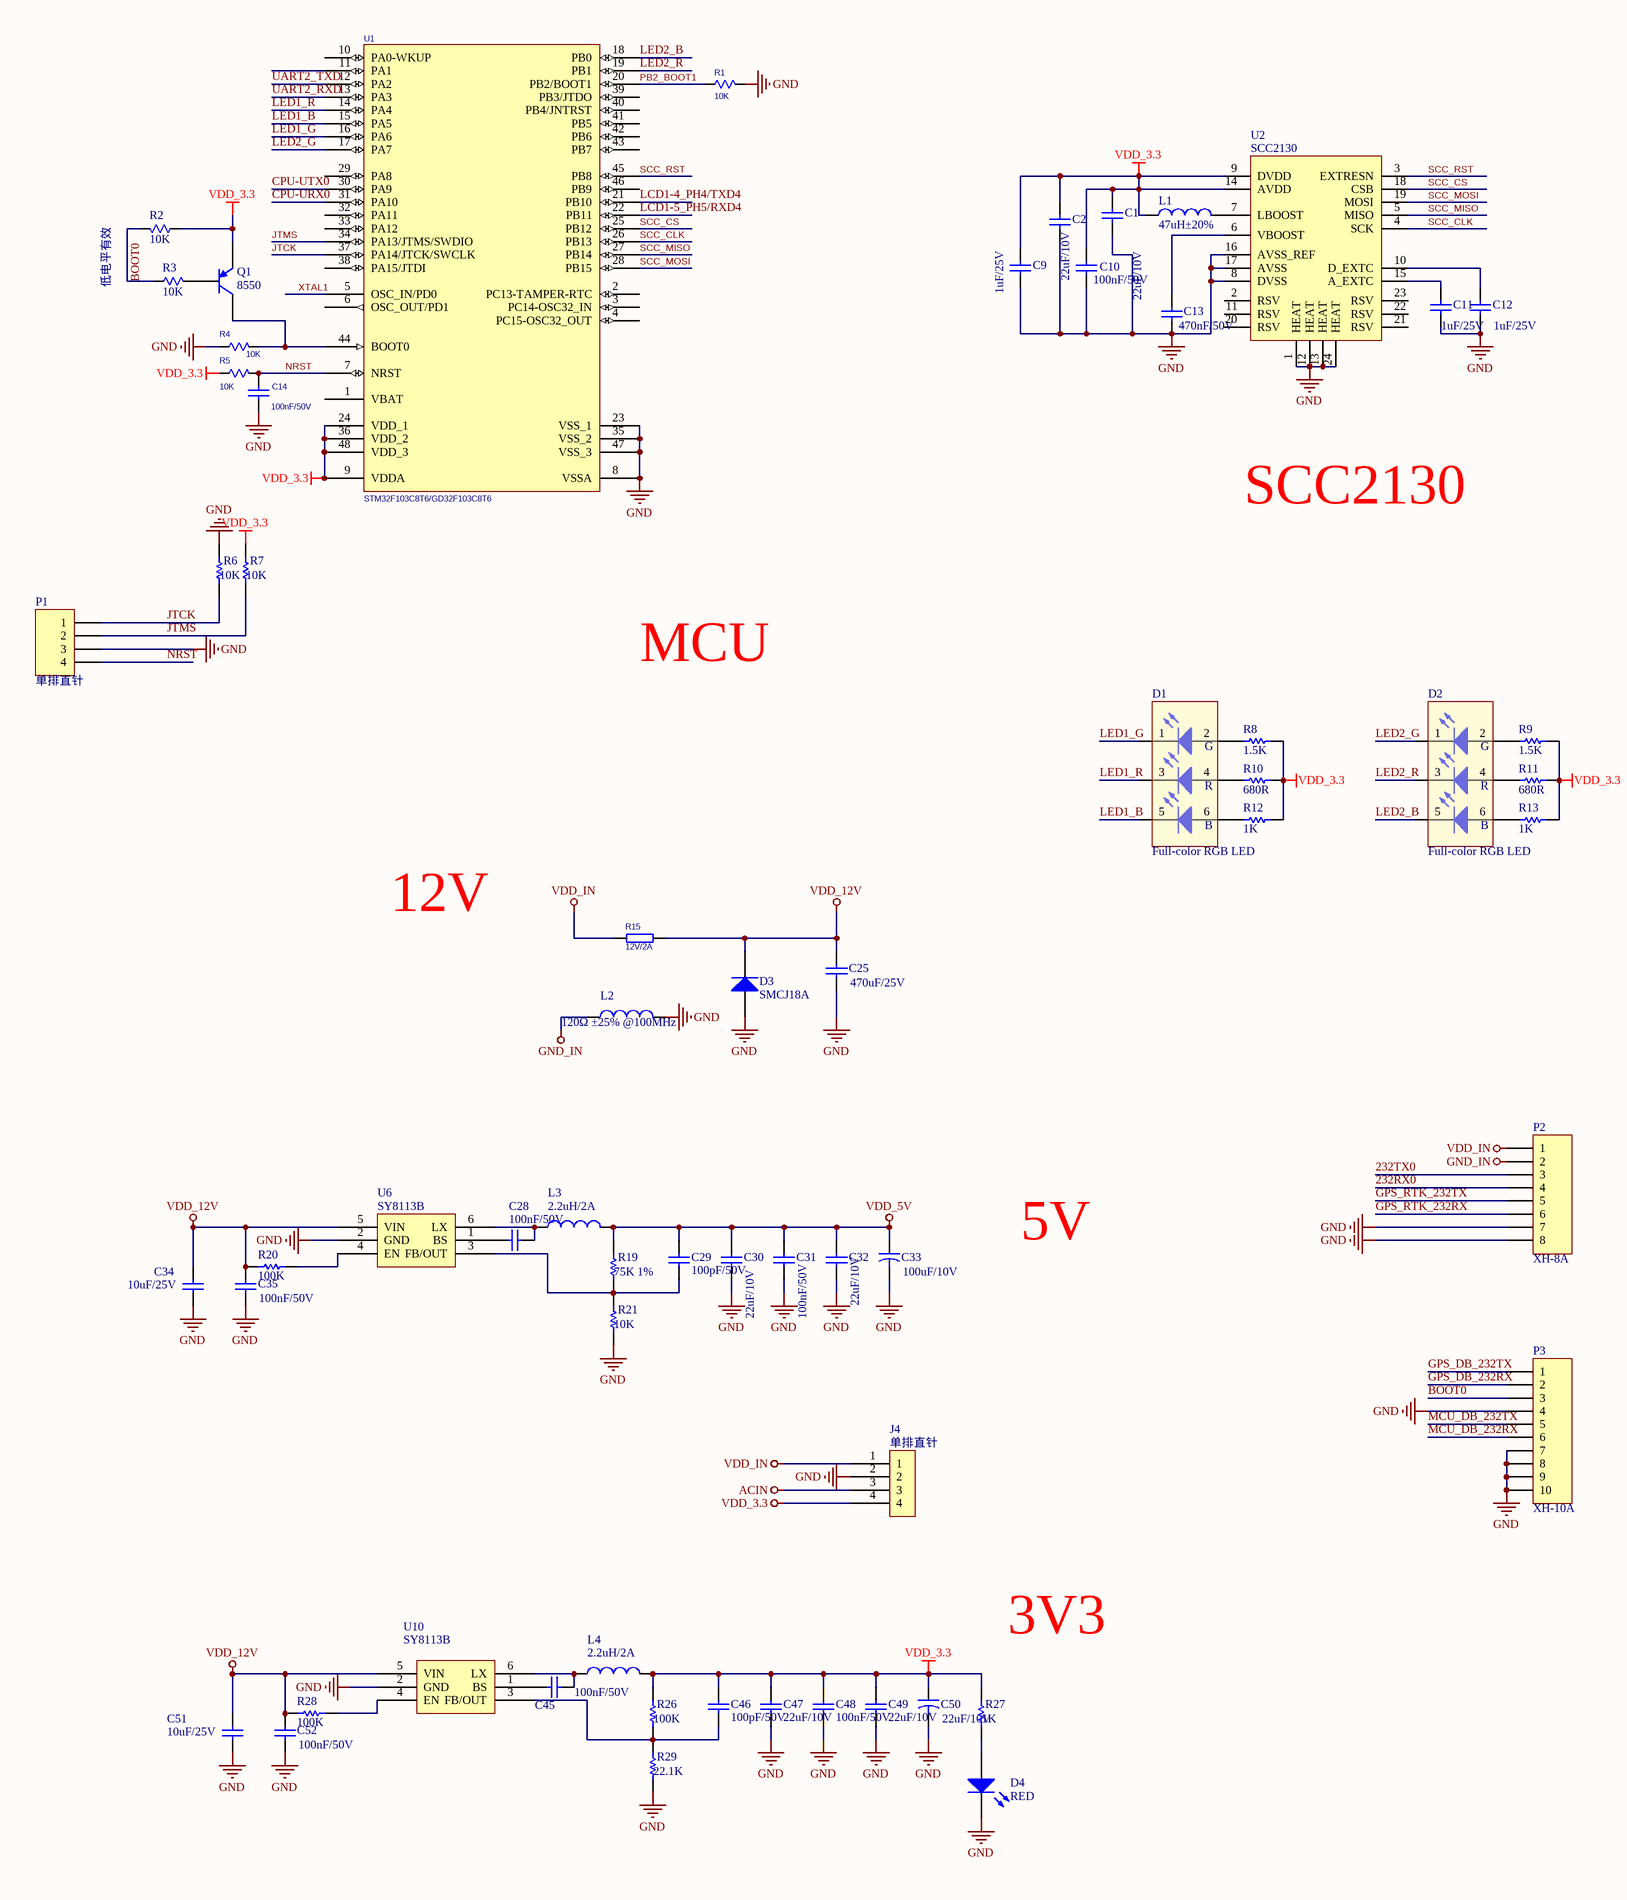
[diagram p0: MISC84436-2.SchDoc, left]
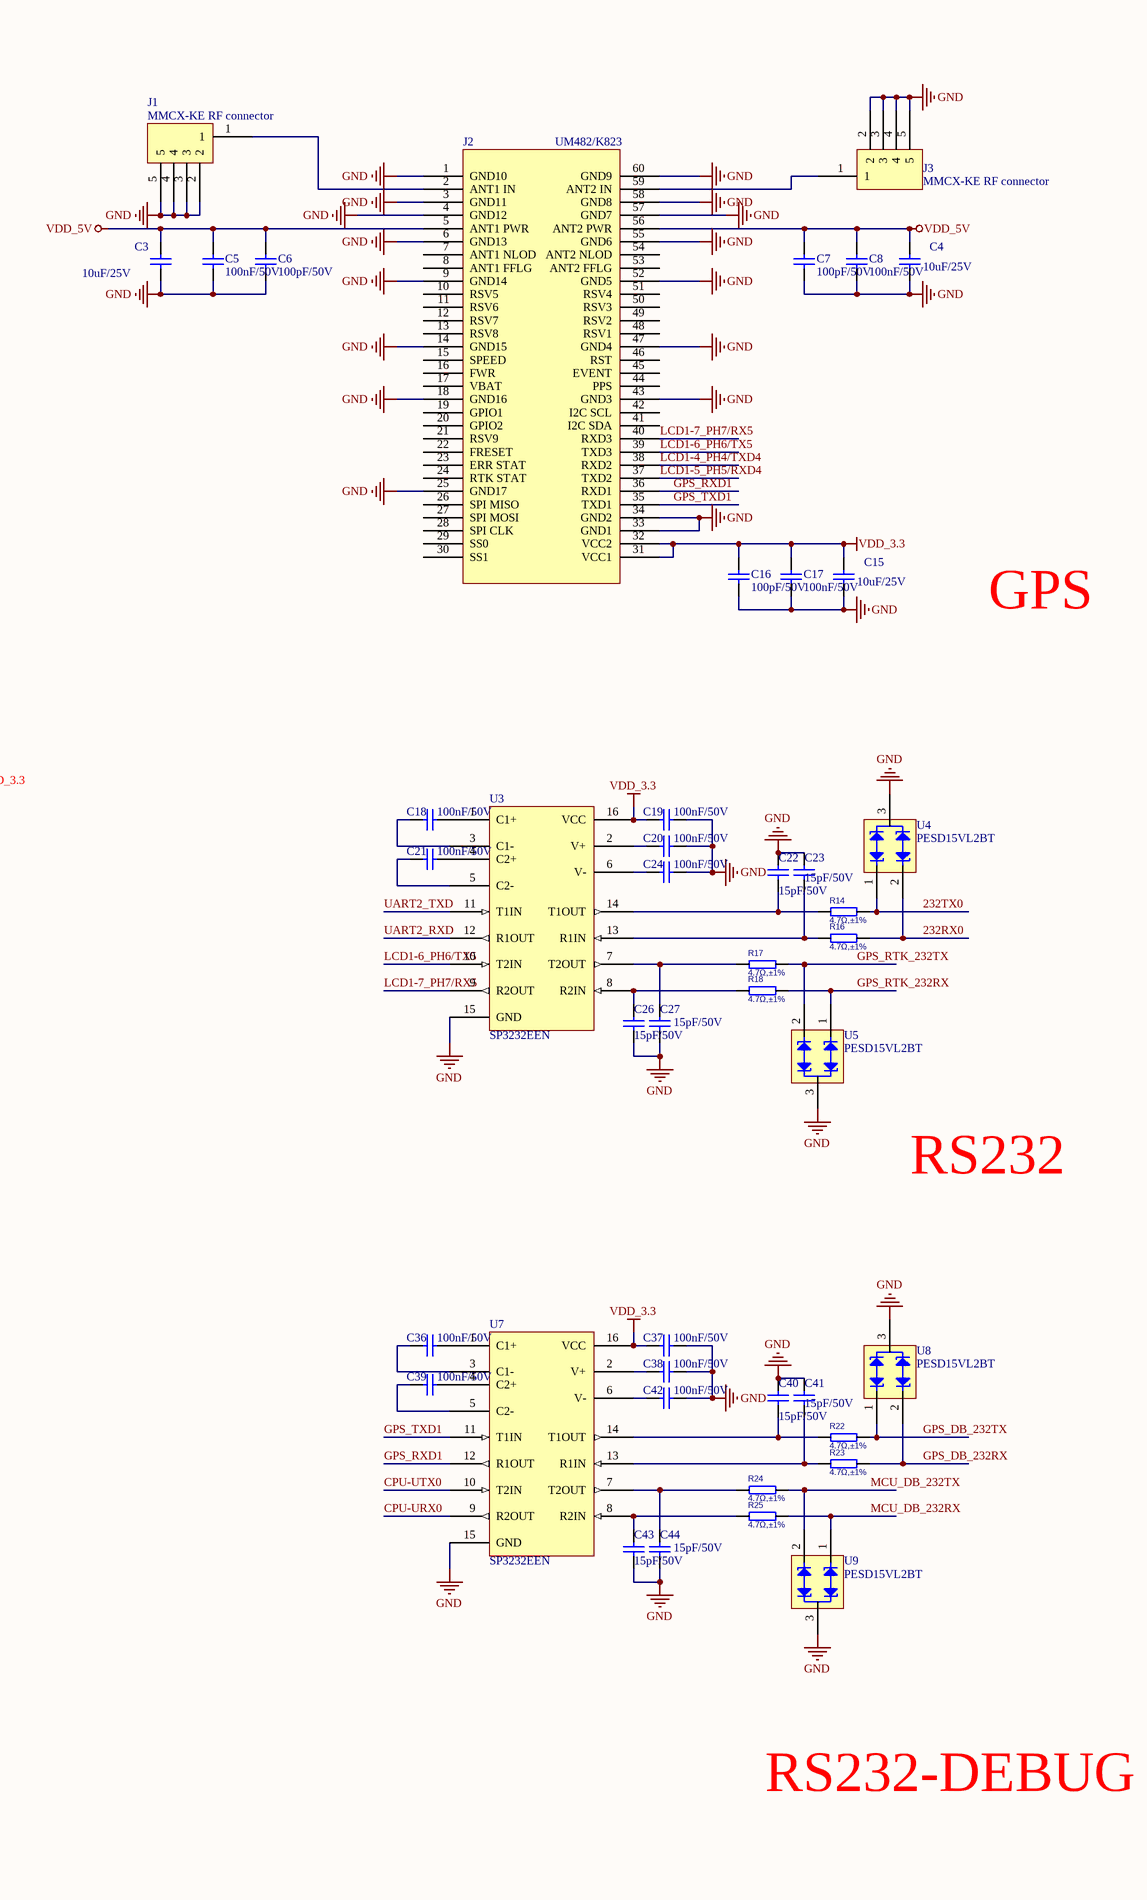
[diagram p1: MISC84436-2.SchDoc, right]
# Altium project MISC84436-3.PrjPcb
1 sheet, 107 parts. Net scope: global (net labels, ports and power ports of the same name join across sheets).
Board file: MISC84436.PcbDoc

## Sheet MISC84436-2.SchDoc
size A2

### Parts
C1  22uF/10V  [C0805]
C2  22uF/10V  [C0805]
C3  10uF/25V  [C0805]
C4  10uF/25V  [C0805]
C5  100nF/50V  [0603]
C6  100pF/50V  [0603]
C7  100pF/50V  [0603]
C8  100nF/50V  [0603]
C9  1uF/25V  [0603]
C10  100nF/50V  [0603]
C11  1uF/25V  [0603]
C12  1uF/25V  [0603]
C13  470nF/50V  [0603]
C14  100nF/50V  [0603]
C15  10uF/25V  [C0805]
C16  100pF/50V  [0603]
C17  100nF/50V  [0603]
C18  100nF/50V  [0603]
C19  100nF/50V  [0603]
C20  100nF/50V  [0603]
C21  100nF/50V  [0603]
C22  15pF/50V  [0603]
C23  15pF/50V  [0603]
C24  100nF/50V  [0603]
C25  470uF/25V  [CAP-TH_BD8.0-P3.50-D1.0-FD]
C26  15pF/50V  [0603]
C27  15pF/50V  [0603]
C28  100nF/50V  [0603]
C29  100pF/50V  [0603]
C30  22uF/10V  [C0805]
C31  100nF/50V  [0603]
C32  22uF/10V  [C0805]
C33  100uF/10V  [CAP-TH_BD5.0-P2.00-D0.8-FD]
C34  10uF/25V  [C0805]
C35  100nF/50V  [0603]
C36  100nF/50V  [0603]
C37  100nF/50V  [0603]
C38  100nF/50V  [0603]
C39  100nF/50V  [0603]
C40  15pF/50V  [0603]
C41  15pF/50V  [0603]
C42  100nF/50V  [0603]
C43  15pF/50V  [0603]
C44  15pF/50V  [0603]
C45  100nF/50V  [0603]
C46  100pF/50V  [0603]
C47  22uF/10V  [C0805]
C48  100nF/50V  [0603]
C49  22uF/10V  [C0805]
C50  22uF/10V  [C0805]
C51  10uF/25V  [C0805]
C52  100nF/50V  [0603]
D1  Full-color RGB LED  [RGB]
D2  Full-color RGB LED  [RGB]
D3  SMCJ18A  [SMC_L6.9-W5.9-LS7.9-RD]
D4  RED  [LED_0805]
J1  MMCX-KE RF connector  [MMCX-TH_ZC11.801KK]
J2  UM482/K823  [UM482/K823]
J3  MMCX-KE RF connector  [MMCX-TH_ZC11.801KK]
J4  单排直针  [HDR1X4]
L1  47uH±20%  [1210]
L2  120Ω ±25% @100MHz  [0603]
L3  2.2uH/2A  [IND-SMD_L4.0-W4.0]
L4  2.2uH/2A  [IND-SMD_L4.0-W4.0]
P1  单排直针  [HDR1X4]
P2  XH-8A  [CONN-TH_XH-8A]
P3  XH-10A  [CONN-TH_10P-P2.50_XH-10A]
Q1  8550  [SOT-23-SS8550]
R1  10K  [0603]
R2  10K  [0603]
R3  10K  [0603]
R4  10K  [0603]
R5  10K  [0603]
R6  10K  [0603]
R7  10K  [0603]
R8  1.5K  [0603]
R9  1.5K  [0603]
R10  680R  [0603]
R11  680R  [0603]
R12  1K  [0603]
R13  1K  [0603]
R14  4.7Ω,±1%  [0603]
R15  12V/2A  [1210]
R16  4.7Ω,±1%  [0603]
R17  4.7Ω,±1%  [0603]
R18  4.7Ω,±1%  [0603]
R19  75K 1%  [0603]
R20  100K  [0603]
R21  10K  [0603]
R22  4.7Ω,±1%  [0603]
R23  4.7Ω,±1%  [0603]
R24  4.7Ω,±1%  [0603]
R25  4.7Ω,±1%  [0603]
R26  100K  [0603]
R27  1K  [0603]
R28  100K  [0603]
R29  22.1K  [0603]
U1  STM32F103C8T6/GD32F103C8T6  [LQFP-48_L7.0-W7.0-P0.50-LS9.0-BL]
U2  SCC2130  [SCC2130D]
U3  SP3232EEN  [SOP16-6.6]
U4  PESD15VL2BT  [SOT-23]
U5  PESD15VL2BT  [SOT-23]
U6  SY8113B  [TSOT-23-6_L2.9-W1.6-P0.95-LS2.8-BR]
U7  SP3232EEN  [SOP16-6.6]
U8  PESD15VL2BT  [SOT-23]
U9  PESD15VL2BT  [SOT-23]
U10  SY8113B  [TSOT-23-6_L2.9-W1.6-P0.95-LS2.8-BR]

### Nets
ACIN: J4.3
GND: C1.2 C2.2 C3.1 C4.1 C5.2 C6.2 C7.1 C8.1 C9.2 C10.2 C11.2 C12.2 C13.2 C14.1 C15.1 C16.1 C17.1 C19.2 C20.2 C22.1 C23.1 C24.2 C25.2 C26.2 C27.2 C30.2 C31.2 C32.2 C33.2 C34.1 C35.1 C37.2 C38.2 C40.1 C41.1 C42.2 C43.2 C44.2 C47.2 C48.2 C49.2 C50.2 C51.1 C52.1 D3.1(A) D4.2(K) J1.2 J1.3 J1.4 J1.5 J2.1(GND10) J2.3(GND11) J2.4(GND12) J2.6(GND13) J2.9(GND14) J2.14(GND15) J2.18(GND16) J2.25(GND17) J2.33(GND1) J2.34(GND2) J2.43(GND3) J2.47(GND4) J2.52(GND5) J2.55(GND6) J2.57(GND7) J2.58(GND8) J2.60(GND9) J3.2 J3.3 J3.4 J3.5 J4.2 L2.2 P1.3 P2.7 P2.8 P3.4 P3.7 P3.8 P3.9 P3.10 R1.1 R4.1 R6.2 R21.1 R29.1 U1.8(VSSA) U1.23(VSS_1) U1.35(VSS_2) U1.47(VSS_3) U2.1(HEAT) U2.8(DVSS) U2.12(HEAT) U2.13(HEAT) U2.16(AVSS_REF) U2.17(AVSS) U2.24(HEAT) U3.15(GND) U4.3 U5.3 U6.2(GND) U7.15(GND) U8.3 U9.3 U10.2(GND)
GND_IN: L2.1 P2.2
VDD_3.3: C1.1 C2.1 C9.1 C10.1 C15.2 C16.2 C17.2 C19.1 C37.1 C46.1 C47.1 C48.1 C49.1 C50.1 J2.31(VCC1) J2.32(VCC2) J4.4 L1.1 L4.2 Q1.2(E) R2.2 R5.2 R7.2 R8.1 R9.1 R10.1 R11.1 R12.1 R13.1 R26.2 R27.2 U1.9(VDDA) U1.24(VDD_1) U1.36(VDD_2) U1.48(VDD_3) U2.9(DVDD) U2.14(AVDD) U3.16(VCC) U7.16(VCC)
VDD_5V: C3.2 C4.2 C5.1 C6.1 C7.2 C8.2 C29.1 C30.1 C31.1 C32.1 C33.1 J2.5(ANT1_PWR) J2.56(ANT2_PWR) L3.2 R19.2
VDD_12V: C25.1 C34.2 C35.2 C51.2 C52.2 D3.2(K) R15.1 R20.2 R28.2 U6.5(VIN) U10.5(VIN)
VDD_IN: J4.1 P2.1 R15.2
232RX0: P2.4 R16.1 U4.2
232TX0: P2.3 R14.1 U4.1
BOOT0: P3.3 R2.1 R3.2
CPU-URX0: U1.31(PA10) U7.9(R2OUT)
CPU-UTX0: U1.30(PA9) U7.10(T2IN)
GPS_DB_232RX: P3.2 R23.1 U8.2
GPS_DB_232TX: P3.1 R22.1 U8.1
GPS_RTK_232RX: P2.6 R18.1 U5.1
GPS_RTK_232TX: P2.5 R17.1 U5.2
GPS_RXD1: J2.36(RXD1) U7.12(R1OUT)
GPS_TXD1: J2.35(TXD1) U7.11(T1IN)
JTCK: P1.1 R6.1 U1.37(PA14/JTCK/SWCLK)
JTMS: P1.2 R7.1 U1.34(PA13/JTMS/SWDIO)
LCD1-4_PH4/TXD4: J2.38(RXD2) U1.21(PB10)
LCD1-5_PH5/RXD4: J2.37(TXD2) U1.22(PB11)
LCD1-6_PH6/TX5: J2.39(TXD3) U3.10(T2IN)
LCD1-7_PH7/RX5: J2.40(RXD3) U3.9(R2OUT)
LED1_B: D1.5(K) U1.15(PA5)
LED1_G: D1.1(K) U1.16(PA6)
LED1_R: D1.3(K) U1.14(PA4)
LED2_B: D2.5(K) U1.18(PB0)
LED2_G: D2.1(K) U1.17(PA7)
LED2_R: D2.3(K) U1.19(PB1)
MCU_DB_232RX: P3.6 R25.1 U9.1
MCU_DB_232TX: P3.5 R24.1 U9.2
NRST: C14.2 P1.4 R5.1 U1.7(NRST)
PB2_BOOT1: R1.2 U1.20(PB2/BOOT1)
SCC_CLK: U1.26(PB13) U2.4(SCK)
SCC_CS: U1.25(PB12) U2.18(CSB)
SCC_MISO: U1.27(PB14) U2.5(MISO)
SCC_MOSI: U1.28(PB15) U2.19(MOSI)
SCC_RST: U1.45(PB8) U2.3(EXTRESN)
UART2_RXD: U1.13(PA3) U3.12(R1OUT)
UART2_TXD: U1.12(PA2) U3.11(T1IN)
XTAL1: U1.5(OSC_IN/PD0)
NetC11_1: C11.1 U2.15(A_EXTC)
NetC12_1: C12.1 U2.10(D_EXTC)
NetC13_1: C13.1 U2.6(VBOOST)
NetC18_1: C18.1 U3.3(C1-)
NetC18_2: C18.2 U3.1(C1+)
NetC20_1: C20.1 U3.2(V+)
NetC21_1: C21.1 U3.5(C2-)
NetC21_2: C21.2 U3.4(C2+)
NetC22_2: C22.2 R14.2 U3.14(T1OUT)
NetC23_2: C23.2 R16.2 U3.13(R1IN)
NetC24_1: C24.1 U3.6(V-)
NetC26_1: C26.1 R18.2 U3.8(R2IN)
NetC27_1: C27.1 R17.2 U3.7(T2OUT)
NetC28_1: C28.1 L3.1 U6.6(LX)
NetC28_2: C28.2 U6.1(BS)
NetC29_2: C29.2 R19.1 R21.2 U6.3(FB/OUT)
NetC36_1: C36.1 U7.3(C1-)
NetC36_2: C36.2 U7.1(C1+)
NetC38_1: C38.1 U7.2(V+)
NetC39_1: C39.1 U7.5(C2-)
NetC39_2: C39.2 U7.4(C2+)
NetC40_2: C40.2 R22.2 U7.14(T1OUT)
NetC41_2: C41.2 R23.2 U7.13(R1IN)
NetC42_1: C42.1 U7.6(V-)
NetC43_1: C43.1 R25.2 U7.8(R2IN)
NetC44_1: C44.1 R24.2 U7.7(T2OUT)
NetC45_1: C45.1 L4.1 U10.6(LX)
NetC45_2: C45.2 U10.1(BS)
NetC46_2: C46.2 R26.1 R29.2 U10.3(FB/OUT)
NetD1_2: D1.2(A) R8.2
NetD1_4: D1.4(A) R10.2
NetD1_6: D1.6(A) R12.2
NetD2_2: D2.2(A) R9.2
NetD2_4: D2.4(A) R11.2
NetD2_6: D2.6(A) R13.2
NetD4_1: D4.1(A) R27.1
NetJ1_1: J1.1 J2.2(ANT1_IN)
NetJ2_59: J2.59(ANT2_IN) J3.1
NetL1_2: L1.2 U2.7(LBOOST)
NetQ1_1: Q1.1(B) R3.1
NetQ1_3: Q1.3(C) R4.2 U1.44(BOOT0)
NetR20_1: R20.1 U6.4(EN)
NetR28_1: R28.1 U10.4(EN)

Not connected (* = marked no-connect by the designer): J2 7(ANT1_NLOD) 8(ANT1_FFLG) 10(RSV5) 11(RSV6) 12(RSV7) 13(RSV8) 15(SPEED) 16(FWR) 17(VBAT) 19(GPIO1) 20(GPIO2) 21(RSV9) 22(FRESET) 23(ERR_STAT) 24(RTK_STAT) 26(SPI_MISO) 27(SPI_MOSI) 28(SPI_CLK) 29(SS0) 30(SS1) 41(I2C_SDA) 42(I2C_SCL) 44(PPS) 45(EVENT) 46(RST) 48(RSV1) 49(RSV2) 50(RSV3) 51(RSV4) 53(ANT2_FFLG) 54(ANT2_NLOD); U1 1(VBAT) 2(PC13-TAMPER-RTC) 3(PC14-OSC32_IN) 4(PC15-OSC32_OUT) 6(OSC_OUT/PD1) 10(PA0-WKUP) 11(PA1) 29(PA8) 32(PA11) 33(PA12) 38(PA15/JTDI) 39(PB3/JTDO) 40(PB4/JNTRST) 41(PB5) 42(PB6) 43(PB7) 46(PB9); U2 2(RSV) 11(RSV) 20(RSV) 21(RSV) 22(RSV) 23(RSV)

### Notes on the sheet
- 低电平有效
- SCC2130
- GPS
- MCU
- 12V
- RS232
- 5V
- 3V3
- RS232-DEBUG

### Library data of the parts
C1 C2 C30 C32 = Cap: SMD ceramic capacitor,X5R; Published: 8-Jun-2000; LatestRevisionDate: 17-Jul-2002; LatestRevisionNote: Re-released for DXP Platform.; PackageReference: RAD-0.3; Value: 22uF/10V; Publisher: Altium Limited
C3 C4 C9-C13 C15 = Cap: SMD ceramic capacitor,X7R; Published: 8-Jun-2000; Publisher: Altium Limited
  C3 C4 C15: LatestRevisionDate: 17-Jul-2002; LatestRevisionNote: Re-released for DXP Platform.; PackageReference: RAD-0.3; Value: 10uF/25V
  C9 C11 C12: Revision: July-2002: Re-released for DXP Platform.; Value: 1uF/25V
  C10: Revision: July-2002: Re-released for DXP Platform.; Value: 100nF/50V
  C13: Revision: July-2002: Re-released for DXP Platform.; Value: 470nF/50V
C5-C8 C16 C17 C28 C29 C31 C35 = Cap: 表贴陶瓷电容; Published: 8-Jun-2000; LatestRevisionDate: 17-Jul-2002; LatestRevisionNote: Re-released for DXP Platform.; PackageReference: RAD-0.3; Publisher: Altium Limited
  C5 C8 C17 C28 C31 C35: Value: 100nF/50V
  C6 C7 C16 C29: Value: 100pF/50V
C14 C45-C49 C51 C52 = Cap: Capacitor; Published: 8-Jun-2000; Publisher: Altium Limited
  C14: Revision: July-2002: Re-released for DXP Platform.; Value: 100nF/50V
  C45 C48 C52: LatestRevisionDate: 17-Jul-2002; LatestRevisionNote: Re-released for DXP Platform.; PackageReference: RAD-0.3; Value: 100nF/50V
  C46: LatestRevisionDate: 17-Jul-2002; LatestRevisionNote: Re-released for DXP Platform.; PackageReference: RAD-0.3; Value: 100pF/50V
  C47 C49: LatestRevisionDate: 17-Jul-2002; LatestRevisionNote: Re-released for DXP Platform.; PackageReference: RAD-0.3; Value: 22uF/10V
  C51: LatestRevisionDate: 17-Jul-2002; LatestRevisionNote: Re-released for DXP Platform.; PackageReference: RAD-0.3; Value: 10uF/25V
C18-C24 C26 C27 C36-C44 = Cap: SMD capacitor,X7R; Published: 8-Jun-2000; Revision: July-2002: Re-released for DXP Platform.; Publisher: Altium Limited
  C18-C21 C24 C36-C39 C42: Value: 100nF/50V
  C22 C23 C26 C27 C40 C41 C43 C44: Value: 15pF/50V
C25 = Cap: 470μF,25V,Ф8×11.5mm,RoHS; Published: 8-Jun-2000; LatestRevisionDate: 17-Jul-2002; LatestRevisionNote: Re-released for DXP Platform.; PackageReference: RAD-0.3; Value: 470uF/25V; Publisher: Altium Limited
C33 = Cap2: 100μF,10V,Ф5×7mm,RoHS; Published: 23-Sep-2002; PackageReference: CAPR5-4X5; Value: 100uF/10V; Publisher: Altium Limited
C34 = Cap: SMD ceramic capacitor,MLCC; Published: 8-Jun-2000; LatestRevisionDate: 17-Jul-2002; LatestRevisionNote: Re-released for DXP Platform.; PackageReference: RAD-0.3; Value: 10uF/25V; Publisher: Altium Limited
C50 = Cap2: Capacitor; Published: 23-Sep-2002; PackageReference: CAPR5-4X5; Value: 22uF/10V; Publisher: Altium Limited
D1 D2 = LED1_3: 19-337C/RSBHGHC-M03/2T,EVERLIGHT (Taiwan); Published: 8-Jun-2000; LatestRevisionDate: 08-Jul-2005; LatestRevisionNote: Mech Layer 1 removed.; PackageReference: LED-1; Publisher: Altium Limited
D3 = Diode: TVS diode; Published: 8-Jun-2000; LatestRevisionDate: 17-Jul-2002; LatestRevisionNote: Re-released for DXP Platform.; PackageVersion: Sep-1996; PackageReference: SMC; Code_JEDEC: DO-214-AB; Publisher: Altium Limited
D4 = LED1: Red high-brightness LED; Published: 8-Jun-2000; LatestRevisionDate: 08-Jul-2005; LatestRevisionNote: Mech Layer 1 removed.; PackageReference: LED-1; Publisher: Altium Limited
J1 J3 = CIRCLE
J2 = UM482: 高精度卫星接收机
J4 = 2.54: Single-row straight header,4P,2.54mm
L1 = Inductor: 表贴电感; Code_IEC: 1005; Published: 8-Jun-2000; LatestRevisionDate: 29-May-2009; LatestRevisionNote: IPC-7351 Footprint Added.; PackageReference: 0402-A; PackageDescription: Chip Inductor; Code_JEITA: 0402; Value: 47uH±20%; Publisher: Altium Limited
L2 = Inductor: 磁珠; Code_IEC: 1005; Published: 8-Jun-2000; LatestRevisionDate: 29-May-2009; LatestRevisionNote: IPC-7351 Footprint Added.; PackageReference: 0402-A; PackageDescription: Chip Inductor; Code_JEITA: 0402; Publisher: Altium Limited
L3 L4 = Inductor: SMD power inductor,cjiang,FNR4026S2R2MT; Code_IEC: 1005; Published: 8-Jun-2000; LatestRevisionDate: 29-May-2009; LatestRevisionNote: IPC-7351 Footprint Added.; PackageReference: 0402-A; PackageDescription: Chip Inductor; Code_JEITA: 0402; Value: 2.2uH/2A; Publisher: Altium Limited
P1 = Header 4: Single-row straight header,4P,2.54mm; LatestRevisionDate: 17-Jul-2002; LatestRevisionNote: Re-released for DXP Platform.; Publisher: Altium Limited
P2 = Header 8: 8P,pitch 2.5mm,through-hole,BOOMELE; LatestRevisionDate: 17-Jul-2002; LatestRevisionNote: Re-released for DXP Platform.; Publisher: Altium Limited
P3 = Header 10: 10P,pitch 2.5mm,through-hole,BOOMELE; LatestRevisionDate: 17-Jul-2002; LatestRevisionNote: Re-released for DXP Platform.; Publisher: Altium Limited
Q1 = PNP: PNP Bipolar Transistor; Published: 8-Jun-2000; LatestRevisionDate: 29-May-2009; LatestRevisionNote: IPC-7351 Footprint Added.; PackageVersion: Aug-1999; PackageReference: SOT-23B; PackageDescription: 3-Pin SOT-23 Package 0.95 mm Pitch, 2.4 mm Lead Span; Publisher: Altium Limited
R1 R4 R5 = Res: 表贴电阻; Published: 8-Jun-2000; LatestRevisionDate: 04-Mar-2005; LatestRevisionNote: PCB Footprint replaced.; PackageReference: J1-0603; Value: 10K; Publisher: Altium Limited
R2 R3 = Res: 标贴电阻; Published: 8-Jun-2000; LatestRevisionDate: 04-Mar-2005; LatestRevisionNote: PCB Footprint replaced.; PackageReference: J1-0603; Value: 10K; Publisher: Altium Limited
R6-R13 R19-R21 R26-R29 = Res1: 表贴电阻; Published: 8-Jun-2000; LatestRevisionDate: 17-Jul-2002; LatestRevisionNote: Re-released for DXP Platform.; PackageReference: AXIAL-0.3; Publisher: Altium Limited
  R6 R7 R21: Value: 10K
  R8 R9: Value: 1.5K
  R10 R11: Value: 680R
  R12 R13 R27: Value: 1K
  R19: Value: 75K 1%
  R20 R26 R28: Value: 100K
  R29: Value: 22.1K
R14 R16-R18 R22-R25 = RES: 表贴电阻; Value: 4.7Ω,±1%
R15 = RES: 自恢复保险丝
U1 = STM32F103C8T6: STM32 ARM-based 32-bit MCU with ST/GD GigaDevice; Published: 30-May-2008; DatasheetVersion: rev6, Mar-2008; PackageVersion: Mar-2008; PackageReference: LQFP48; PackageDescription: 48-Pin Low-Profile Quad Flat Pack, 7 x 7 mm Body, 0.5 mm Pitch (LQFP48); ComponentLink1Description: Manufacturer Link; ComponentLink1URL: www.st.com/stm32; ComponentLink2Description: Datasheet; ComponentLink2URL: http://www.st.com/stonline/products/literature/ds/13587.pdf; Publisher: Altium Limited
U2 = SCC2130: MEMS digital gyroscope
U3 U7 = SP202ECT
U4 U5 U8 U9 = PESD12VL2BT